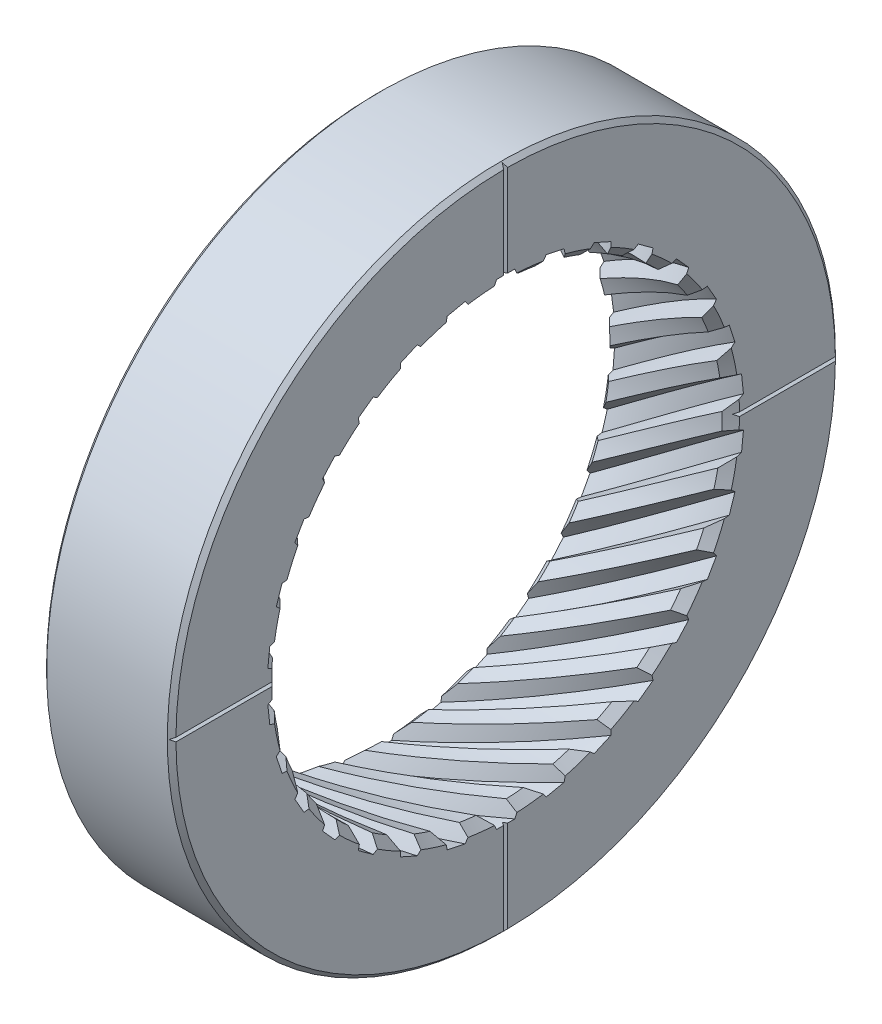
from build123d import *

# Parameters (mm, degrees)
SKETCH_1_R               = 77.5
SKETCH_1_R_2             = 52.25
EXTRUDE_1_DEPTH          = 30
CHAMFER_2_SIZE           = 2
CHAMFER_1_SIZE           = 1
SWEEP_3_PITCH            = 480
SWEEP_3_HEIGHT           = 30
SWEEP_3_RADIUS           = 53.5
SWEEP_3_START_ANGLE      = -90
PATTERN_CIRCULAR_4_COUNT = 30
CUT_EXTRUDE_2_DEPTH      = 176.872823387
PATTERN_CIRCULAR_6_COUNT = 4


with BuildPart() as part:
    # 草图1 → 凸台-拉伸1 (new body)
    with BuildSketch(Plane(origin=(0, 0, 0), x_dir=(0, 0, -1), z_dir=(1, 0, 0))):
        Circle(SKETCH_1_R)
        Circle(SKETCH_1_R_2, mode=Mode.SUBTRACT)
    extrude(amount=EXTRUDE_1_DEPTH)

    # 倒角2
    chamfer_2_edges = [part.edges().sort_by_distance(p)[0] for p in [
        (0, 0, 52.25),
        (30, 0, 52.25),
    ]]
    chamfer(chamfer_2_edges, length=CHAMFER_2_SIZE)

    # 倒角1
    chamfer_1_edges = [part.edges().sort_by_distance(p)[0] for p in [
        (0, 0, 77.5),
        (30, 0, 77.5),
    ]]
    chamfer(chamfer_1_edges, length=CHAMFER_1_SIZE)

    # 切除-扫描3: sweep along a helix
    with BuildLine() as sweep_3_path:
        add(Helix(SWEEP_3_PITCH, SWEEP_3_HEIGHT, SWEEP_3_RADIUS, center=(30, 0, 0), direction=(-1, 0, 0), mode=Mode.PRIVATE).rotate(Axis((30, 0, 0), (-1, 0, 0)), SWEEP_3_START_ANGLE))
    # Sketch 556 → 切除-扫描3 (sweep, cut)
    with BuildSketch(Plane(origin=(30, 0, 0), x_dir=(0, 0, -1), z_dir=(1, 0, 0))):
        Polygon((-2.120849801, 55.25), (-3.679150199, 51.75), (3.679150199, 51.75), (2.120849801, 55.25), align=None)
    sweep_3 = sweep(path=sweep_3_path.line, is_frenet=True, mode=Mode.SUBTRACT)

    # 阵列(圆周)4: 切除-扫描3 ×30 about axis
    pattern_circular_4_axis = Axis((30, 0, 0), (-1, 0, 0))
    for i in range(1, PATTERN_CIRCULAR_4_COUNT):
        add(sweep_3.rotate(pattern_circular_4_axis, i * 360 / PATTERN_CIRCULAR_4_COUNT), mode=Mode.SUBTRACT)

    # 草图6 → 切除-拉伸2 (cut, through all)
    with BuildSketch(Plane(origin=(0, 77.5, 0), x_dir=(1, 0, 0), z_dir=(0, 1, 0))):
        Polygon((0.8, 0), (0, 0.461880215), (0, -0.461880215), align=None)
        Polygon((29.2, 0), (30, -0.461880215), (30, 0.461880215), align=None)
    cut_extrude_2 = extrude(amount=-CUT_EXTRUDE_2_DEPTH, mode=Mode.SUBTRACT)

    # 阵列(圆周)6: 切除-拉伸2 ×4 about axis
    pattern_circular_6_axis = Axis((30, 0, 0), (-1, 0, 0))
    for i in range(1, PATTERN_CIRCULAR_6_COUNT):
        add(cut_extrude_2.rotate(pattern_circular_6_axis, i * 360 / PATTERN_CIRCULAR_6_COUNT), mode=Mode.SUBTRACT)


solid = part.part
